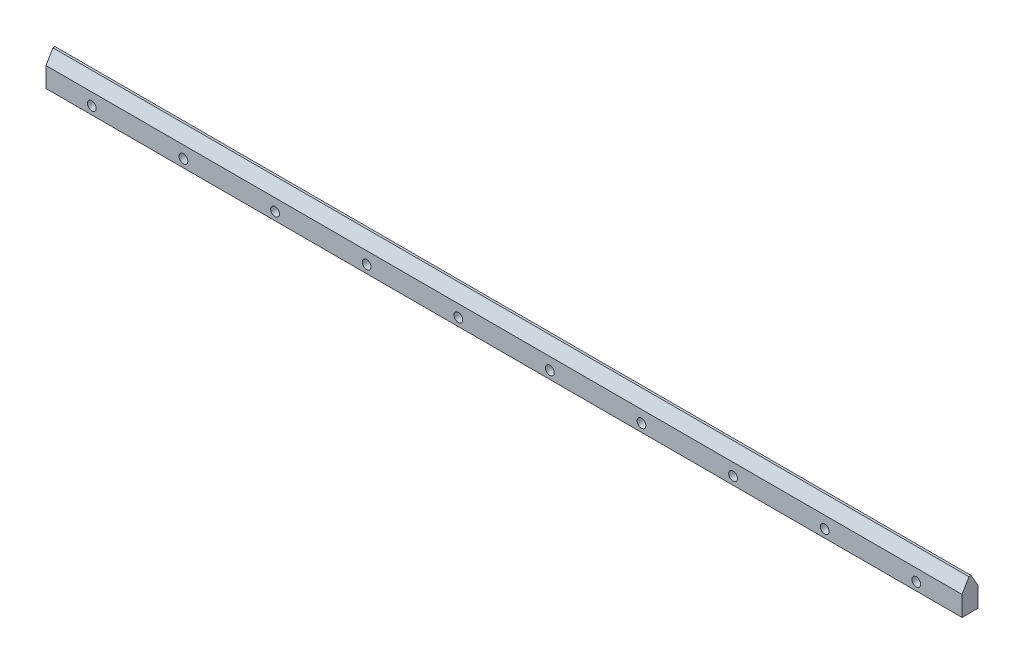
SolidWorks part; units mm, degrees
ref_plane "Front Plane" through (0, 0, 0) normal (0, 0, 1) x (1, 0, 0)
ref_plane "Top Plane" through (0, 0, 0) normal (0, 1, 0) x (1, 0, 0)
ref_plane "Right Plane" through (0, 0, 0) normal (1, 0, 0) x (0, 0, -1)
sketch "Sketch1" plane through (0, 0, 0) normal (1, 0, 0) x (0, 0, -1)
  line L0 (-2.6795, 40) -> (-20, 10)
  line L1 (-2.6795, 40) -> (2.6795, 40)
  line L2 (-20, 10) -> (-20, -40)
  line L3 (-20, -40) -> (20, -40)
  line L4 (20, 10) -> (20, -40)
  line L5 (-20, 40) -> (20, -40) construction
  line L6 (-20, -40) -> (20, 40) construction
  line L7 (2.6795, 40) -> (20, 10)
  point P0 (0, 0)
  dimension "D1" = 40
  dimension "D2" = 80
  dimension "D3" = 60
  dimension "D4" = 60
  dimension "D5" = 30
  dimension "D6" = 30
extrude "Boss-Extrude1" add sketch "Sketch1" along normal blind 2300
sketch "Sketch2" plane through (0, 0, 20) normal (0, 0, 1) x (1, 0, 0)
  line L0 (0, 10) -> (0, -40) construction
  line L1 (2300, -40) -> (0, -40) construction
  circle A0 centre (115, -20) radius 5
  dimension "D1" = 10
  dimension "D2" = 115
  dimension "D3" = 20
extrude "Cut-Extrude1" cut sketch "Sketch2" against normal through all
sketch "Sketch3" plane through (0, 0, 20) normal (0, 0, 1) x (1, 0, 0)
  circle A0 centre (115, -20) radius 11
  dimension "D1" = 22
extrude "Cut-Extrude2" cut sketch "Sketch3" against normal blind 20
pattern_linear "LPattern1" count 10 spacing 230 along (1, 0, 0) of "Cut-Extrude2", "Cut-Extrude1"
